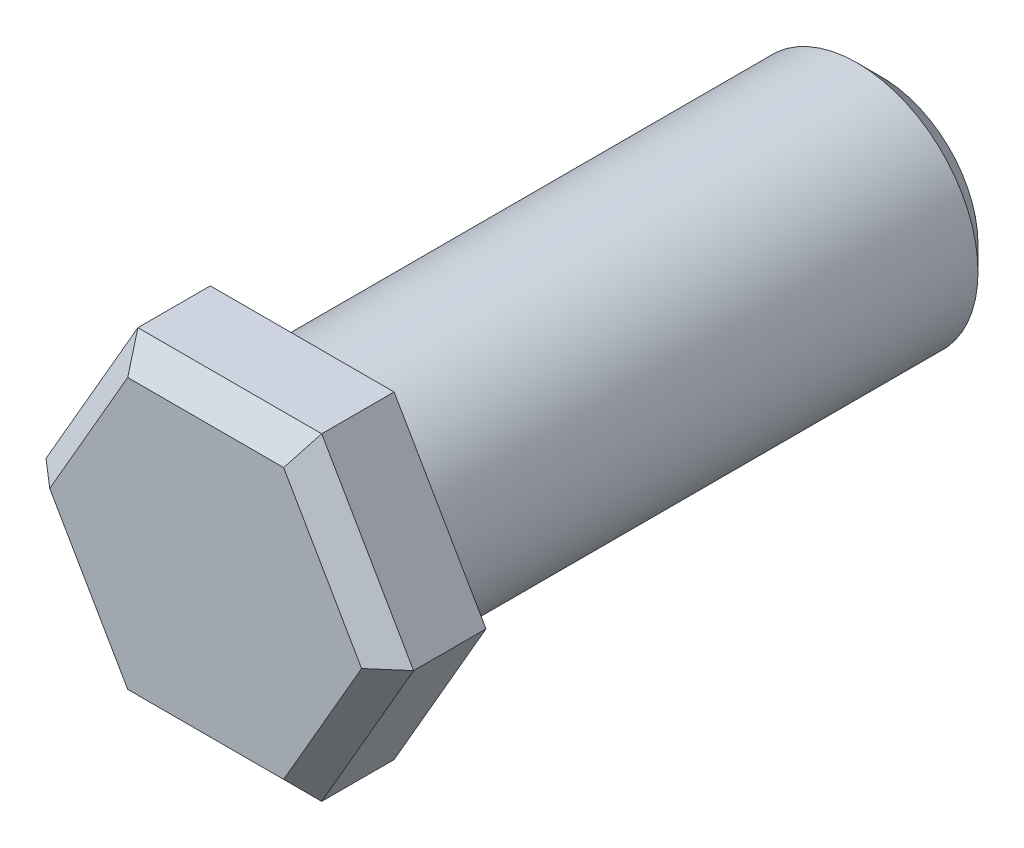
SolidWorks part; units mm, degrees
ref_plane "Front Plane" through (0, 0, 0) normal (0, 0, 1) x (1, 0, 0)
ref_plane "Top Plane" through (0, 0, 0) normal (0, 1, 0) x (1, 0, 0)
ref_plane "Right Plane" through (0, 0, 0) normal (1, 0, 0) x (0, 0, -1)
sketch "Sketch1" plane through (0, 0, 0) normal (0, 0, 1) x (1, 0, 0)
  circle A0 centre (720, 45) radius 2.5 construction
  circle A1 centre (720, 45) radius 2.5
extrude "Boss-Extrude1" add sketch "Sketch1" against normal blind 12
sketch "Sketch2" plane through (0, 0, 0) normal (0, 0, 1) x (1, 0, 0)
  line L1 (718.0961, 41.7023) -> (721.9039, 41.7023)
  line L2 (721.9039, 41.7023) -> (723.8078, 45)
  line L3 (723.8078, 45) -> (721.9039, 48.2977)
  line L4 (721.9039, 48.2977) -> (718.0961, 48.2977)
  line L5 (718.0961, 48.2977) -> (716.1922, 45)
  line L6 (716.1922, 45) -> (718.0961, 41.7023)
  circle A0 centre (720, 45) radius 3.2977 construction
extrude "Boss-Extrude2" add sketch "Sketch2" along normal blind 2
chamfer "Chamfer1" distance 0.5 angle 45 7 edges at (722.5, 45, -12) (717.1441, 46.6488, 2) (720, 48.2977, 2) (722.8559, 46.6488, 2) (722.8559, 43.3512, 2) (720, 41.7023, 2) (717.1441, 43.3512, 2)
